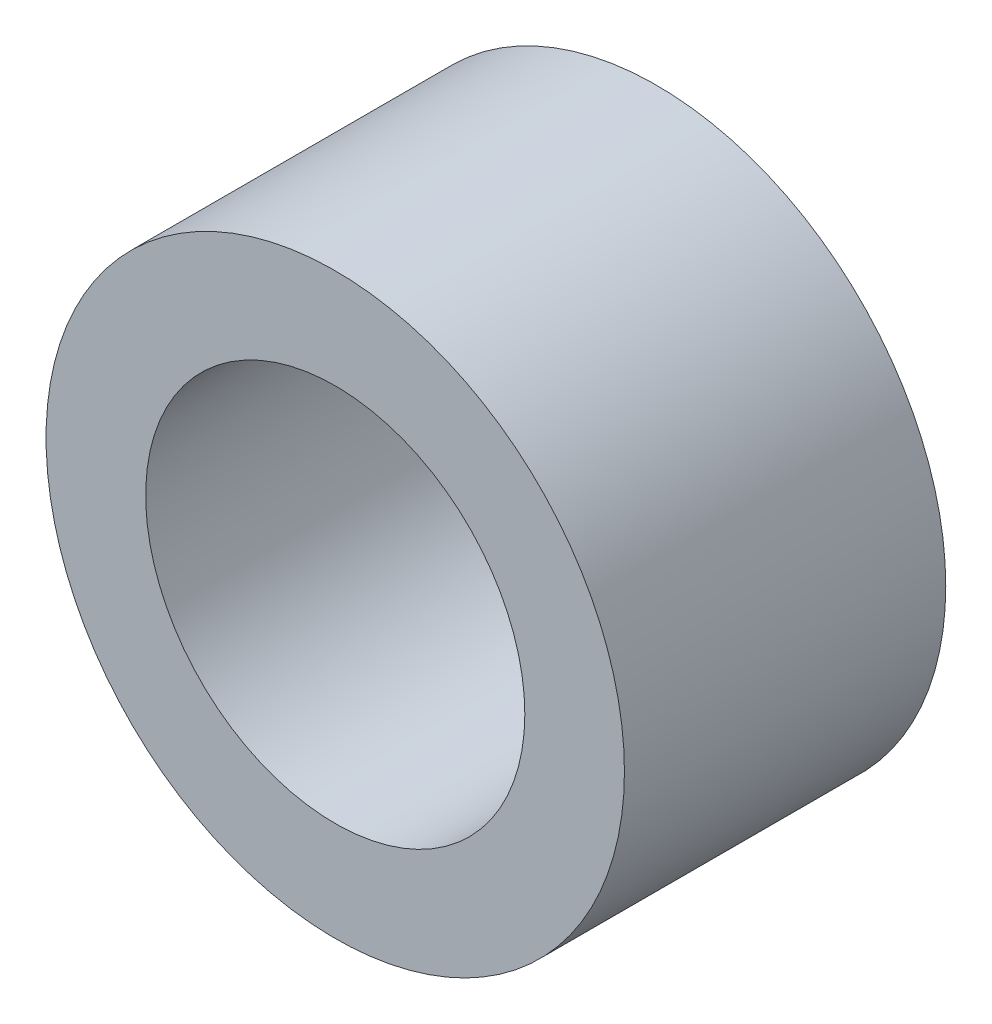
SolidWorks part; units mm, degrees
ref_plane "Front Plane" through (0, 0, 0) normal (0, 0, 1) x (1, 0, 0)
ref_plane "Top Plane" through (0, 0, 0) normal (0, 1, 0) x (1, 0, 0)
ref_plane "Right Plane" through (0, 0, 0) normal (1, 0, 0) x (0, 0, -1)
sketch "Sketch1" plane through (0, 0, 0) normal (0, 0, 1) x (1, 0, 0)
  circle A0 centre (0, 0) radius 22.5
  circle A1 centre (0, 0) radius 14.75
extrude "Boss-Extrude1" add sketch "Sketch1" along normal blind 25
